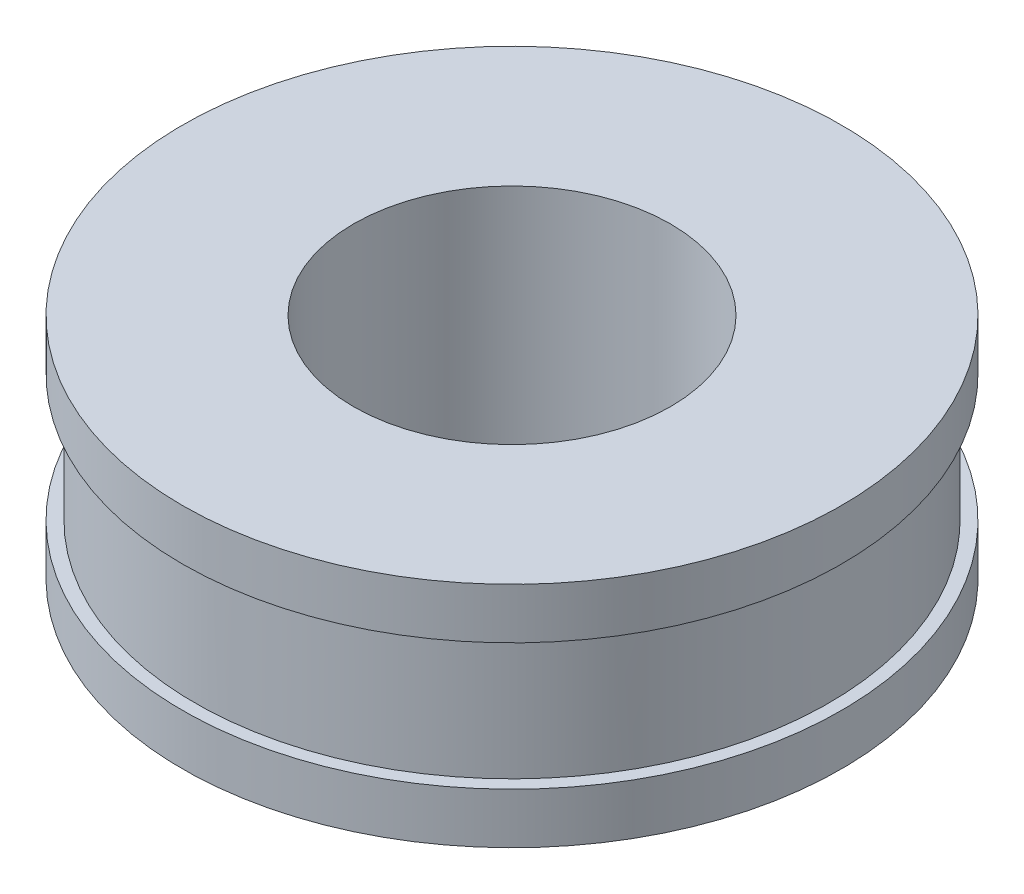
SolidWorks part; units mm, degrees
ref_plane "Front Plane" through (0, 0, 0) normal (0, 0, 1) x (1, 0, 0)
ref_plane "Top Plane" through (0, 0, 0) normal (0, 1, 0) x (1, 0, 0)
ref_plane "Right Plane" through (0, 0, 0) normal (1, 0, 0) x (0, 0, -1)
sketch "Sketch1" plane through (0, 0, 0) normal (0, 1, 0) x (1, 0, 0)
  circle A0 centre (0, 0) radius 50
extrude "Boss-Extrude1" add sketch "Sketch1" along normal blind 20
sketch "Sketch2" plane through (0, 20, 0) normal (0, 1, 0) x (1, 0, 0)
  circle A0 centre (0, 0) radius 52
extrude "Boss-Extrude2" add sketch "Sketch2" along normal blind 8
sketch "Sketch3" plane through (0, 0, 0) normal (0, -1, 0) x (1, 0, 0)
  circle A0 centre (0, 0) radius 52
extrude "Boss-Extrude3" add sketch "Sketch3" along normal blind 8
sketch "Sketch4" plane through (0, -8, 0) normal (0, -1, 0) x (1, 0, 0)
  circle A0 centre (0, 0) radius 25
extrude "Cut-Extrude1" cut sketch "Sketch4" against normal through all
